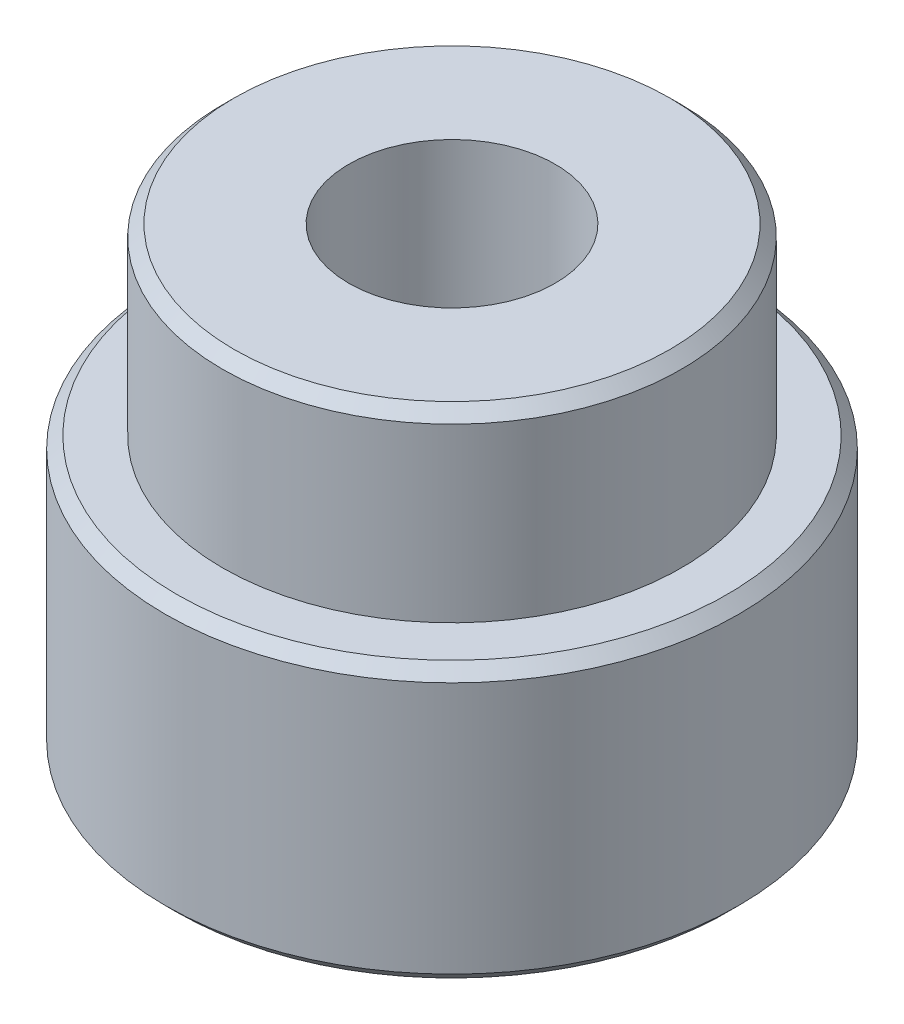
from build123d import *

# Parameters (mm, degrees)
SKETCH_1_R          = 10
EXTRUDE_1_DEPTH     = 20
SKETCH_3_R          = 12.5
EXTRUDE_2_DEPTH     = 12
SKETCH_2_R          = 4.5
CUT_EXTRUDE_1_DEPTH = 27.69269563
CHAMFER_2_SIZE      = 0.5


with BuildPart() as part:
    # 草图1 → 凸台-拉伸1 (new body)
    with BuildSketch(Plane(origin=(0, 0, 0), x_dir=(1, 0, 0), z_dir=(0, 1, 0))):
        with Locations(Location((0, 0, 0), (0, 0, 270))):
            Circle(SKETCH_1_R)
    extrude(amount=EXTRUDE_1_DEPTH)

    # 草图3 → 凸台-拉伸2 (add)
    with BuildSketch(Plane(origin=(0, 0, 0), x_dir=(-1, 0, 0), z_dir=(0, -1, 0))):
        with Locations(Location((0, 0, 0), (0, 0, 90))):
            Circle(SKETCH_3_R)
    extrude(amount=-EXTRUDE_2_DEPTH)

    # 草图2 → 切除-拉伸1 (cut, through all)
    with BuildSketch(Plane(origin=(0, 20, 0), x_dir=(1, 0, 0), z_dir=(0, 1, 0))):
        with Locations(Location((0, 0, 0), (0, 0, 270))):
            Circle(SKETCH_2_R)
    extrude(amount=-CUT_EXTRUDE_1_DEPTH, mode=Mode.SUBTRACT)

    # 倒角2
    chamfer_2_edges = [part.edges().sort_by_distance(p)[0] for p in [
        (0, 20, -10),
        (0, 12, 12.5),
        (0, 0, 12.5),
    ]]
    chamfer(chamfer_2_edges, length=CHAMFER_2_SIZE)


solid = part.part
